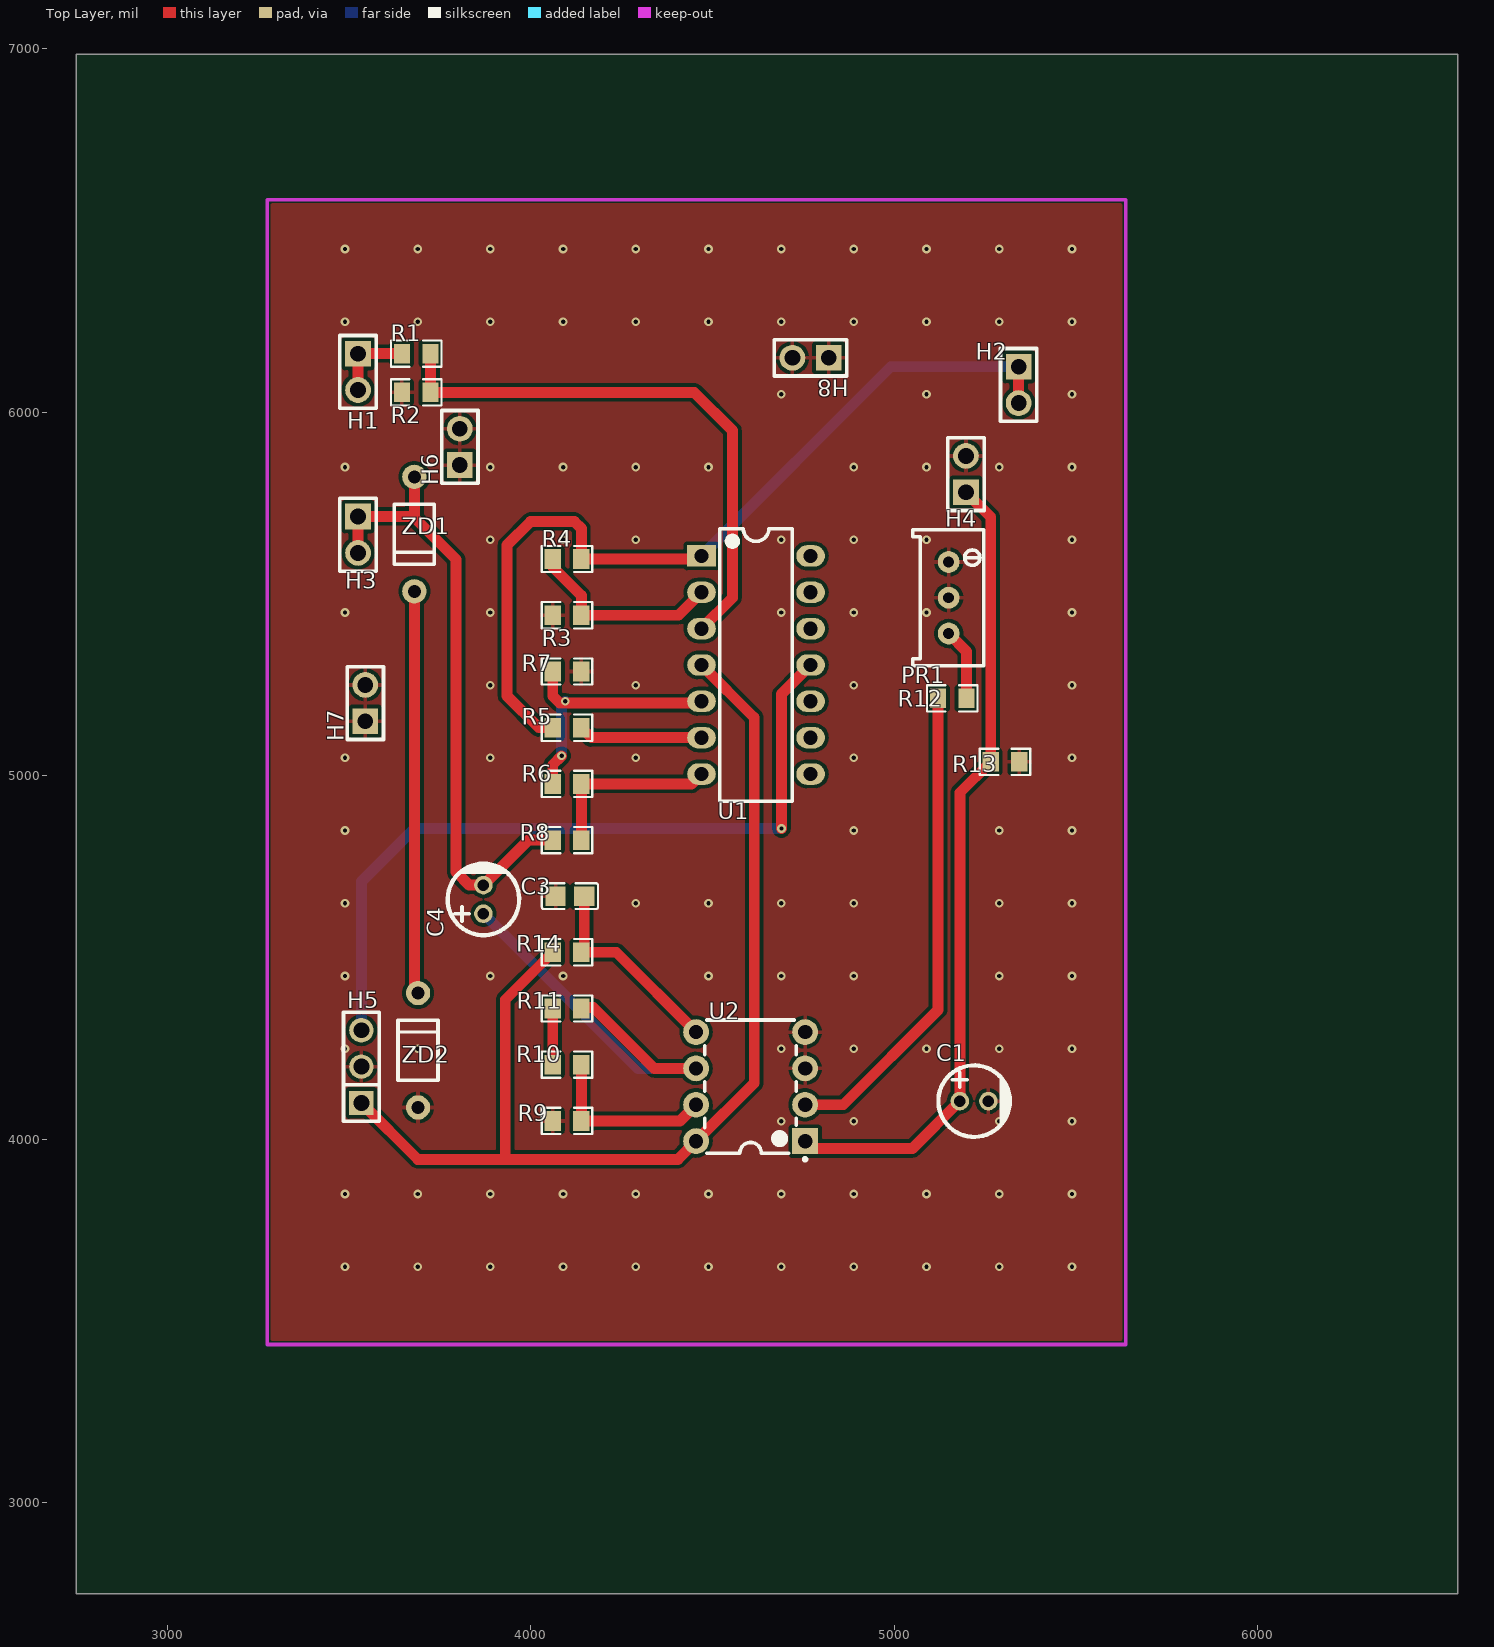
[diagram p0: Top Layer view]
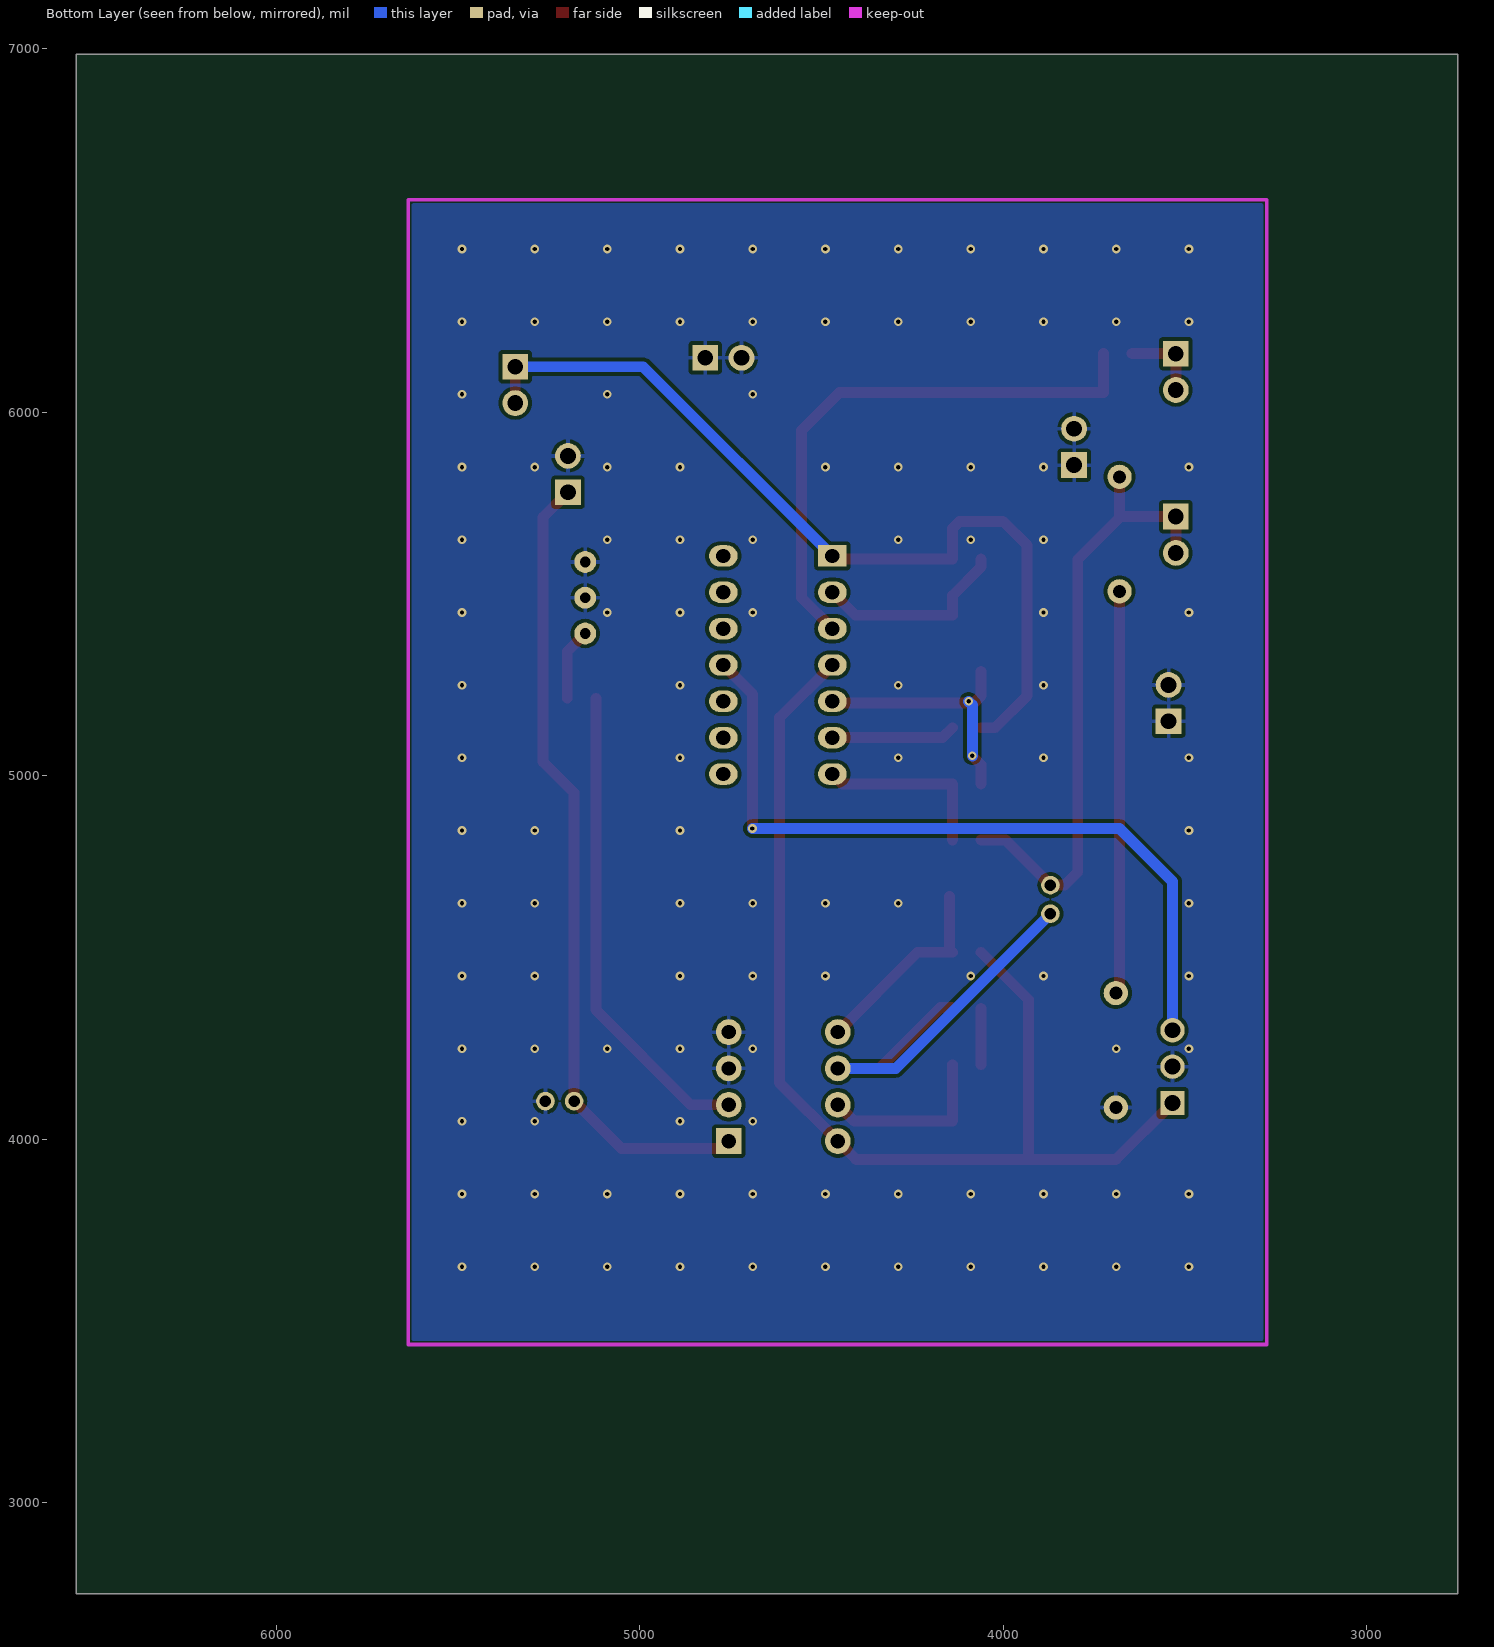
[diagram p1: Bottom Layer view, seen from below]
# Altium PCB MISC51973.pcbdoc
Units mil, origin at the board's own origin, x right, y up, seen from the top; angles counter-clockwise.
Board outline 3800 x 4235 mil, 2 copper layers (Top Layer, Bottom Layer), stack 62.206 mil thick; 30 components, 19 nets, 80 pads, 111 vias.

## Layer stack, top to bottom
Top Solder Mask Layer: solder mask 0.394, Dk 3.3
Top Layer: signal copper 1.379
Dielectric1: surface 59.449, FR4, Dk 4.5
Bottom Layer: signal copper 1.378
Bottom Solder Mask Layer: solder mask 0.394, Dk 3.3

## Board outline
6550,2750 2750,2750 2750,6985 6550,6985

## Design rules (kind name [scope] priority, off if disabled: settings)
BoardOutlineClearance copperThickness2oz_1 [All] p2 off: genericclearance=7.99 ignorepadtopadclearanceinfootprint=FALSE except(0: Arc-SplitContinuation Track-SplitContinuation SMDPad-SplitContinuation THPad-SplitContinuation Via-SplitContinuation Fill-SplitContinuation Region-SplitContinuation Poly-SplitContinuation Text-SplitContinuation Hole-SplitContinuation; 5.98: Arc-CutoutEdge SMDPad-CutoutEdge THPad-CutoutEdge Via-CutoutEdge Fill-CutoutEdge Region-CutoutEdge Text-CutoutEdge; 6.93: Hole-OutlineEdge Hole-CutoutEdge; 10: Poly-OutlineEdge Poly-CutoutEdge; 11.81: Arc-OutlineEdge Track-OutlineEdge SMDPad-OutlineEdge THPad-OutlineEdge Via-OutlineEdge Fill-OutlineEdge Region-OutlineEdge Text-OutlineEdge Track-CutoutEdge)
BoardOutlineClearance copperThickness1oz_1 [All] p4: genericclearance=4.02 ignorepadtopadclearanceinfootprint=FALSE except(0: Arc-SplitContinuation Track-SplitContinuation SMDPad-SplitContinuation THPad-SplitContinuation Via-SplitContinuation Fill-SplitContinuation Region-SplitContinuation Poly-SplitContinuation Text-SplitContinuation Hole-SplitContinuation; 6: SMDPad-CutoutEdge THPad-CutoutEdge Via-CutoutEdge Fill-CutoutEdge Region-CutoutEdge Text-CutoutEdge; 6.93: Hole-OutlineEdge Hole-CutoutEdge; 10: Poly-OutlineEdge Poly-CutoutEdge; 11.8: Arc-OutlineEdge Track-OutlineEdge SMDPad-OutlineEdge THPad-OutlineEdge Via-OutlineEdge Fill-OutlineEdge Region-OutlineEdge Text-OutlineEdge; 11.81: Arc-CutoutEdge Track-CutoutEdge)
Clearance copperThickness2oz [All] p1 off: gap=7.99 ignorepadtopadclearanceinfootprint=FALSE except(5.98: SMDPad-Track SMDPad-SMDPad THPad-Track SMDPad-THPad THPad-THPad Track-Via SMDPad-Via THPad-Via Via-Via Fill-Track Region-Track Fill-SMDPad Region-SMDPad Fill-THPad Region-THPad Fill-Via Region-Via Fill-Fill Fill-Region Region-Region Arc-Track Arc-SMDPad Arc-THPad Arc-Via Fill-Arc Region-Arc Arc-Arc Text-Track SMDPad-Text Text-THPad Text-Via Fill-Text Region-Text Arc-Text Text-Text; 6.93: Hole-Track Hole-SMDPad Hole-THPad Hole-Via Fill-Hole Region-Hole Hole-Arc Hole-Text; 10: Poly-Track Poly-SMDPad Poly-THPad Poly-Via Poly-Fill Poly-Region Poly-Poly Poly-Arc Poly-Text Poly-Hole)
Clearance copperThickness1oz [All] p3: gap=4.02 ignorepadtopadclearanceinfootprint=FALSE except(5.98: SMDPad-Track SMDPad-SMDPad THPad-Track SMDPad-THPad THPad-THPad Track-Via SMDPad-Via THPad-Via Via-Via Fill-Track Region-Track Fill-SMDPad Region-SMDPad Fill-THPad Region-THPad Fill-Via Region-Via Fill-Fill Fill-Region Region-Region; 6: Arc-Track Arc-SMDPad Arc-THPad Arc-Via Fill-Arc Region-Arc Arc-Arc Text-Track SMDPad-Text Text-THPad Text-Via Fill-Text Region-Text Arc-Text Text-Text; 6.93: Hole-Track Hole-SMDPad Hole-THPad Hole-Via Fill-Hole Region-Hole Hole-Arc Hole-Text; 10: Poly-Track Poly-SMDPad Poly-THPad Poly-Via Poly-Fill Poly-Region Poly-Poly Poly-Arc Poly-Text Poly-Hole)
DiffPairsRouting differentialPair [All] p1: maxlimit=6 minlimit=6 mostfreqgap=6 toplayer_minwidth=5 toplayer_prefwidth=10 toplayer_maxwidth=100 toplayer_mingap=6 toplayer_prefgap=6 toplayer_maxgap=6 bottomlayer_minwidth=5 bottomlayer_prefwidth=10 bottomlayer_maxwidth=100 bottomlayer_mingap=6 bottomlayer_prefgap=6 bottomlayer_maxgap=6 maxuncoupledlength=10
HoleToHoleClearance otherClearance [All] p1: gap=11.81 allowstackedmicrovias=TRUE
Length netLength [All] p1: minlimit=0 maxlimit=0
MatchedLengths netLengthTolerance [All] p1: tolerance=1000
PasteMaskExpansion pasteMaskExpansion [All] p1: expansion=0
PlaneConnect innerPlane [All] p1: planeconnectstyle=Relief reliefexpansion=20 reliefentries=4 reliefconductorwidth=10 reliefairgap=10
PolygonConnect copperRegion [(InNet('GND'))] p1: connectstyle=Relief reliefconductorwidth=10 reliefentries=4 polygonreliefangle="90 Angle" airgapwidth=10 via.connectstyle=Relief via.reliefconductorwidth=10 via.reliefentries=4 via.polygonreliefangle="90 Angle" via.airgapwidth=10
RoutingVias viaSize [All] p1: holewidth=12.01 width=24.02 viastyle="Through Hole" minholewidth=11.81 minwidth=19.68 maxholewidth=248.03 maxwidth=393.7
SolderMaskExpansion solderMaskExpansion [IsVia] p1: expansion=-1000 istentingtop=TRUE
SolderMaskExpansion solderMaskExpansion [All] p2: expansion=2 istentingtop=FALSE
Width copperThickness2oz_2 [All] p1 off: maxlimit=100 minlimit=8 preferedwidth=10
Width copperThickness1oz_2 [All] p2: maxlimit=100 minlimit=5 preferedwidth=10

## Components (designator, comment, footprint, x,y, rotation, side; value= is the part's Value field where it differs from the comment)
C1 "1uF" CAP-TH_BD5.0-P2.00-D0.8-FD-10UF50VC110GL 5220,4105 r0 top
C3 "0.01uF" C0805 4107.97,4668.82 r0 top
C4 "470pF" CAP-TH_BD5.0-P2.00-D0.8-FD-10UF50VC110GL 3870,4660 r90 top
H1 "" HDR-TH_2P-P2.54-V-M-1 3525,6111.51 r270 top
H2 "" HDR-TH_2P-P2.54-V-M-1 5342.5,6075.57 r270 top
H3 "" HDR-TH_2P-P2.54-V-M-1 3525,5663.26 r270 top
H4 "" HDR-TH_2P-P2.54-V-M-1 5197.5,5830.03 r90 top
H5 "" HDR-TH_3P-P2.54-V-M 3534.21,4200 r90 top
H6 "" HDR-TH_2P-P2.54-V-M-1 3805,5905 r90 top
H7 "" HDR-TH_2P-P2.54-V-M-1 3545,5200 r90 top
H8 "" HDR-TH_2P-P2.54-V-M-1 4770,6150 r180 top
PR1 "5kΩ" R_3296 5155,5490 r270 top
R1 "1K" R0805 3685,6161.51 r0 top
R2 "100K" R0805 3685,6055 r0 top
R3 "1K" R0805 4100,5441.81 r0 top
R4 "10K" R0805 4100,5596.51 r0 top
R5 "1K" R0805 4100,5132.4 r180 top
R6 "100K" R0805 4100,4977.7 r180 top
R7 "1K" R0805 4100,5287.1 r0 top
R8 "1K" R0805 4100,4822.99 r0 top
R9 "68K" R0805 4100,4050.53 r0 top
R10 "10K" R0805 4100,4205.24 r180 top
R11 "100K" R0805 4100,4359.94 r180 top
R12 "12K" R0805 5160,5213.38 r180 top
R13 "100K" R0805 5305,5038.38 r180 top
R14 "6.81K" R0805 4100,4514.64 r180 top
U1 "LM324" PDIP-14_L19.3-W6.5-P2.54-LS7.6-BL 4620,5305 r270 top
U2 "100kHz" DIP-8_L9.2-W6.4-P2.54-LS7.6-BL 4605,4145 r90 top
ZD1 "1N4733A" DO-41_BD2.8-L4.2-P8.00-D0.7-FD 3680,5665 r270 top
ZD2 "1N4733A" DO-41_BD2.8-L4.2-P8.00-D0.7-FD 3690,4245 r90 top

## Footprints (in the part's own frame and the unit in brackets; to place one, negate y for a bottom-side part, rotate by r counter-clockwise, add the part's x,y. Pads: shape width x height; smd on the part's side, far side on the other; paste and mask are expansions set on the pad)
C0805 [mm]
  rect 1.41x1.35 smd paste-100 mask+0.051: 1(-1,0) 2(1,0)
  silkscreen extent -1.96,-0.9 1.96,0.9
CAP-TH_BD5.0-P2.00-D0.8-FD-10UF50VC110GL [mm]
  round 1.3 hole 0.8: 1(-1,0) 2(1,0)
  silkscreen extent -2.5,-2.5 2.5,2.5
DIP-8_L9.2-W6.4-P2.54-LS7.6-BL [mm]
  rect 1.8x1.8 hole 1: 1(-3.81,-3.81)
  round 1.8 hole 1: 2(-1.27,-3.81) 3(1.27,-3.81) 4(3.81,-3.81) 5(3.81,3.81) 6(1.27,3.81) 7(-1.27,3.81) 8(-3.81,3.81)
  silkscreen extent -5.18,-3.91 4.65,3.2
DO-41_BD2.8-L4.2-P8.00-D0.7-FD [mm]
  round 1.7 hole 0.9: 1(-4,0) 2(4,0)
  silkscreen extent -2.1,-1.4 2.1,1.4
HDR-TH_2P-P2.54-V-M-1 [mm]
  rect 1.8x1.8 hole 1.1: 1(-1.27,0)
  round 1.8 hole 1.1: 2(1.27,0)
  silkscreen extent -2.54,-1.27 2.54,1.27
HDR-TH_3P-P2.54-V-M [mm]
  rect 1.7x1.7 hole 1.1: 1(-2.54,0)
  round 1.7 hole 1.1: 2(0,0) 3(2.54,0)
  silkscreen extent -3.81,-1.25 3.81,1.25
PDIP-14_L19.3-W6.5-P2.54-LS7.6-BL [mm]
  rect 1.5x2 hole 1: 1(-7.62,-3.81)
  oval 1.5x2 hole 1: 2(-5.08,-3.81) 3(-2.54,-3.81) 4(0,-3.81) 5(2.54,-3.81) 6(5.08,-3.81) 7(7.62,-3.81) 8(7.62,3.81) 9(5.08,3.81) 10(2.54,3.81) 11(0,3.81) 12(-2.54,3.81) 13(-5.08,3.81) 14(-7.62,3.81)
  silkscreen extent -9.53,-2.55 9.53,2.53
R0805 [mm]
  rect 1.133x1.377 smd paste-100 mask+0.051: 1(-1,0) 2(1,0)
  silkscreen extent -1.76,-0.92 1.76,0.92
R_3296 [mil]
  round 60 hole 30 paste+0 mask+2: 1(-98.4,-5) 2(0,-5) 3(98.4,-5)
  silkscreen extent -187,-103 187,92

## Via types
v1: diameter 24.02, hole 12, Top Layer to Bottom Layer, 111 vias

## Nets (pads, with @x,y where several pads share a name; then routed paths per layer and width w, separated by ;. In a path a pad name is that pad's centre, name@x,y a point inside that pad or via, vN(x,y) a via of type N, cw(c..) or ccw(c..) an arc to the next point about the centre after c; other vN are vias at no path point)
$1N1: R1.2 R2.2 U1.3 | length 1560.8
  Top Layer w30: R1.2 R2.2 4450,6055 4555,5950 4555,5490 U1.3
$1N7: H2.1 H2.2 R4.2 R5.2 U1.1 | length 2422.6
  Top Layer w30: R5.2 4022.6,5132.4 3935,5220 3935,5635 4000,5700 4120,5700 4139.37,5680.63 R4.2 4461.51,5596.51 U1.1 ; H2.2 H2.1
  Bottom Layer w30: U1.1 4990.57,6125.57 H2.1
$1N8: R3.2 R4.1 U1.2 | length 544.1
  Top Layer w30: R4.1 4060.63,5574.37 4139.37,5495.63 R3.2 4406.81,5441.81 U1.2
$1N12: R5.1 U1.6 | length 342
  Top Layer w30: R5.1 4166.77,5105 U1.6
$1N13: R6.2 R7.1 U1.5 | length 728.7
  Top Layer w30: R6.2 4060.63,5030.63 v1(4085,5055) ; R7.1 4060.63,5219.37 4080,5200 4465,5200 U1.5
  Bottom Layer w30: v1(4085,5055) 4085,5195 v1(4095,5205)
$1N15: R6.1 R8.2 U1.7 | length 496.6
  Top Layer w30: R8.2 R6.1 4442.7,4977.7 U1.7
$1N16: C4.2 H3.1 H3.2 R8.1 ZD1.1 | length 1723.1
  Top Layer w30: H3.2 H3.1 3676.74,5713.26 3680,5710 ; ZD1.1 3680,5710 ; R8.1 3993.62,4822.99 C4.2 3830.63,4699.37 3795,4735 3795,5595 3680,5710
$1N18: ZD1.2 ZD2.2 | length 1109.2
  Top Layer w30: ZD1.2 3680,4412.48 ZD2.2
$1N20: C4.1 R11.1 U2.6 | length 1152.4
  Top Layer w30: R11.1@4136,4356.57 4142.22,4362.78 4172.22,4362.78 4340,4195 U2.6
  Bottom Layer w30: C4.1 4295.63,4195 U2.6
$1N23: R10.2 R11.2 | length 154.7
  Top Layer w30: R10.2 R11.2
$1N24: C3.2 R14.1 U2.5 | length 564.1
  Top Layer w30: C3.2 4147.34,4522.62 R14.1 4235.36,4514.64 U2.5
$1N25: R9.2 R10.1 U2.7 | length 488.8
  Top Layer w30: R10.1 R9.2 4410.53,4050.53 U2.7
$1N32: R12.2 U2.2 | length 1331.3
  Top Layer w30: U2.2 4860,4095 5120.63,4355.63 R12.2
$1N33: PR1.3 R12.1 | length 198.7
  Top Layer w30: PR1.3 5199.37,5342.23 R12.1
+15V: H5.1 R14.2 U1.4 U2.8 | length 3065.8
  Top Layer w30: H5.1 3689.21,3945 3930,3945 ; R14.2 3930,4384.01 3930,3945 ; U1.4 4615,5160 4615,4155 U2.8 4405,3945 3930,3945
-15V: H5.3 U1.11 | length 2108.5
  Top Layer w30: v1(4690,4855) 4690,5225 U1.11
  Bottom Layer w30: H5.3 3534.21,4709.21 3680,4855 v1(4690,4855)
GND: C1.2 C3.1 H4.2 H5.2 H6.1 H6.2 H7.1 H7.2 H8.1 H8.2 PR1.1 PR1.2 R2.1 R3.1 R7.2 R9.1 R13.1 U2.3 U2.4 ZD2.1
  other v1: 3489.1,3649.49 3689.1,3649.49 3889.1,3649.49 4089.1,3649.49 4289.1,3649.49 4489.1,3649.49 4689.1,3649.49 4889.1,3649.49 5089.1,3649.49 5289.1,3649.49 5489.1,3649.49 3489.1,3849.49 3689.1,3849.49 3889.1,3849.49 4089.1,3849.49 4289.1,3849.49 4489.1,3849.49 4689.1,3849.49 4889.1,3849.49 5089.1,3849.49 5289.1,3849.49 5489.1,3849.49 4689.1,4049.49 4889.1,4049.49 5289.1,4049.49 5489.1,4049.49 3489.1,4249.49 3689.1,4249.49 4689.1,4249.49 4889.1,4249.49 5089.1,4249.49 5289.1,4249.49 5489.1,4249.49 3489.1,4449.49 3889.1,4449.49 4089.1,4449.49 4489.1,4449.49 4689.1,4449.49 4889.1,4449.49 5289.1,4449.49 5489.1,4449.49 3489.1,4649.49 4289.1,4649.49 4489.1,4649.49 4689.1,4649.49 4889.1,4649.49 5289.1,4649.49 5489.1,4649.49 3489.1,4849.49 4889.1,4849.49 5289.1,4849.49 5489.1,4849.49 3489.1,5049.49 3889.1,5049.49 4289.1,5049.49 4889.1,5049.49 5489.1,5049.49 3889.1,5249.49 4289.1,5249.49 4889.1,5249.49 5489.1,5249.49 3489.1,5449.49 3889.1,5449.49 4689.1,5449.49 4889.1,5449.49 5089.1,5449.49 5489.1,5449.49 3889.1,5649.49 4089.1,5649.49 4289.1,5649.49 4689.1,5649.49 4889.1,5649.49 5089.1,5649.49 5489.1,5649.49 3489.1,5849.49 3889.1,5849.49 4089.1,5849.49 4289.1,5849.49 4489.1,5849.49 4889.1,5849.49 5089.1,5849.49 5289.1,5849.49 5489.1,5849.49 4689.1,6049.49 5089.1,6049.49 5489.1,6049.49 3489.1,6249.49 3689.1,6249.49 3889.1,6249.49 4089.1,6249.49 4289.1,6249.49 4489.1,6249.49 4689.1,6249.49 4889.1,6249.49 5089.1,6249.49 5289.1,6249.49 5489.1,6249.49 3489.1,6449.49 3689.1,6449.49 3889.1,6449.49 4089.1,6449.49 4289.1,6449.49 4489.1,6449.49 4689.1,6449.49 4889.1,6449.49 5089.1,6449.49 5289.1,6449.49 5489.1,6449.49
LIN: H1.1 H1.2 R1.1 | length 220.6
  Top Layer w30: H1.2 H1.1 R1.1
VOUT: C1.1 H4.1 R13.2 U2.1 | length 2226.2
  Top Layer w30: U2.1 4775,3975 5050.63,3975 C1.1 5180.63,4953.38 R13.2 5265.63,5711.9 H4.1
pads on no net: U1.8 U1.9 U1.10 U1.12 U1.13 U1.14

## Polygon pours and split planes (outlines as drawn)
GND on Top Layer (solid, remove dead copper, pour order 0): 3000,6700 3000,3000 6300,3000 6300,6700
GND on Bottom Layer (solid, remove dead copper, pour order 2): 3075,6735 3075,3350 5995,3350 5995,6735

## Keep-outs
Board Outline Layer:
  lines w10: 3275,3435.39 3275,6585 5637.2,6585 5637.2,3435.39 3275,3435.39